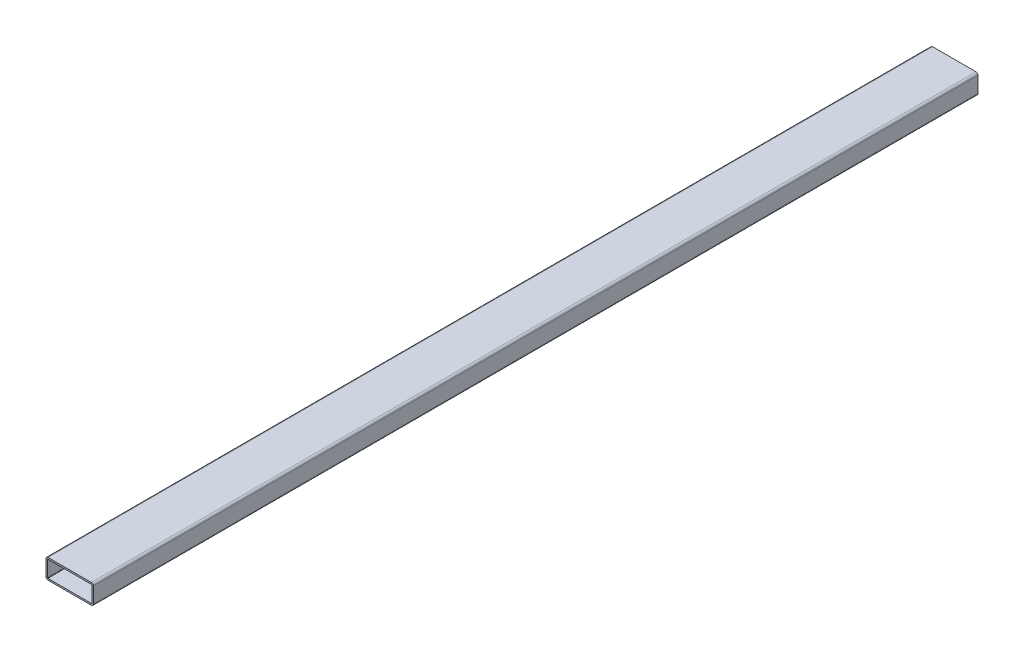
from build123d import *

# Parameters (mm, degrees)
BOSS_EXTRUDE1_DEPTH = 2240
SHELL1_T            = -4


with BuildPart() as part:
    # Sketch1 → Boss-Extrude1 (new body)
    with BuildSketch(Plane.XY):
        with BuildLine():
            Line((55, 25), (-55, 25))
            ThreePointArc((-55, 25), (-58.535533906, 23.535533906), (-60, 20))
            Line((-60, 20), (-60, -20))
            ThreePointArc((-60, -20), (-58.535533906, -23.535533906), (-55, -25))
            Line((-55, -25), (55, -25))
            ThreePointArc((55, -25), (58.535533906, -23.535533906), (60, -20))
            Line((60, -20), (60, 20))
            ThreePointArc((60, 20), (58.535533906, 23.535533906), (55, 25))
        make_face()
    extrude(amount=BOSS_EXTRUDE1_DEPTH)

    # Shell1
    shell1_openings = [part.faces().sort_by_distance(p)[0] for p in [
        (0, 0, 2240),
        (0, 0, 0),
    ]]
    offset(amount=SHELL1_T, openings=shell1_openings, kind=Kind.INTERSECTION)


solid = part.part
